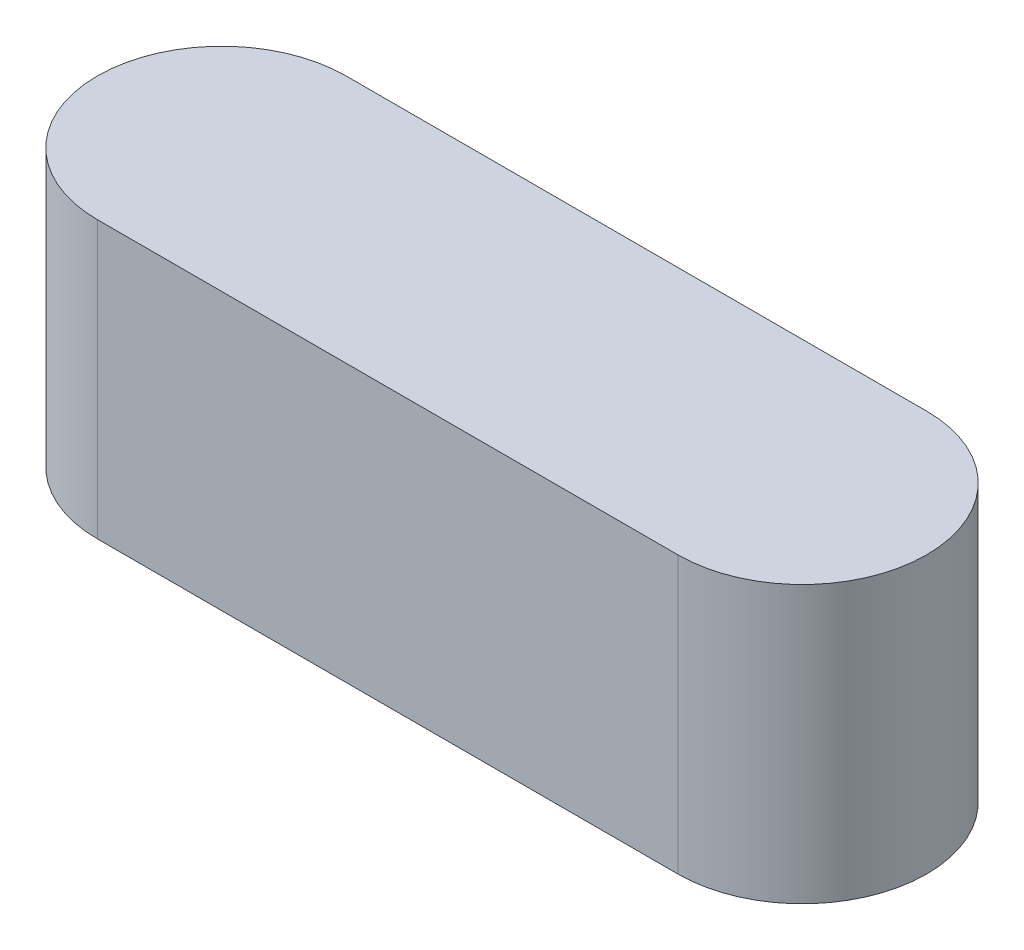
SolidWorks part; units mm, degrees
ref_plane "Front" through (0, 0, 0) normal (0, 0, 1) x (1, 0, 0)
ref_plane "Top" through (0, 0, 0) normal (0, 1, 0) x (1, 0, 0)
ref_plane "Right" through (0, 0, 0) normal (1, 0, 0) x (0, 0, -1)
sketch "Sketch1" plane through (0, 0, 0) normal (0, 1, 0) x (1, 0, 0)
  line L0 (0, 0) -> (21, 0) construction
  line L1 (0, 4.5) -> (21, 4.5)
  line L2 (0, -4.5) -> (21, -4.5)
  arc A0 (0, 4.5) -> (0, -4.5) centre (0, 0) ccw
  arc A1 (21, -4.5) -> (21, 4.5) centre (21, 0) ccw
  point P3 (10.5, 0)
  dimension "D2" = 4.5
  dimension "D1" = 21
extrude "Boss-Extrude1" add sketch "Sketch1" along normal blind 10
scale "Scale 1" bodies to scale 101 scale about centroid uniform scaling yes scale factor 1.875
